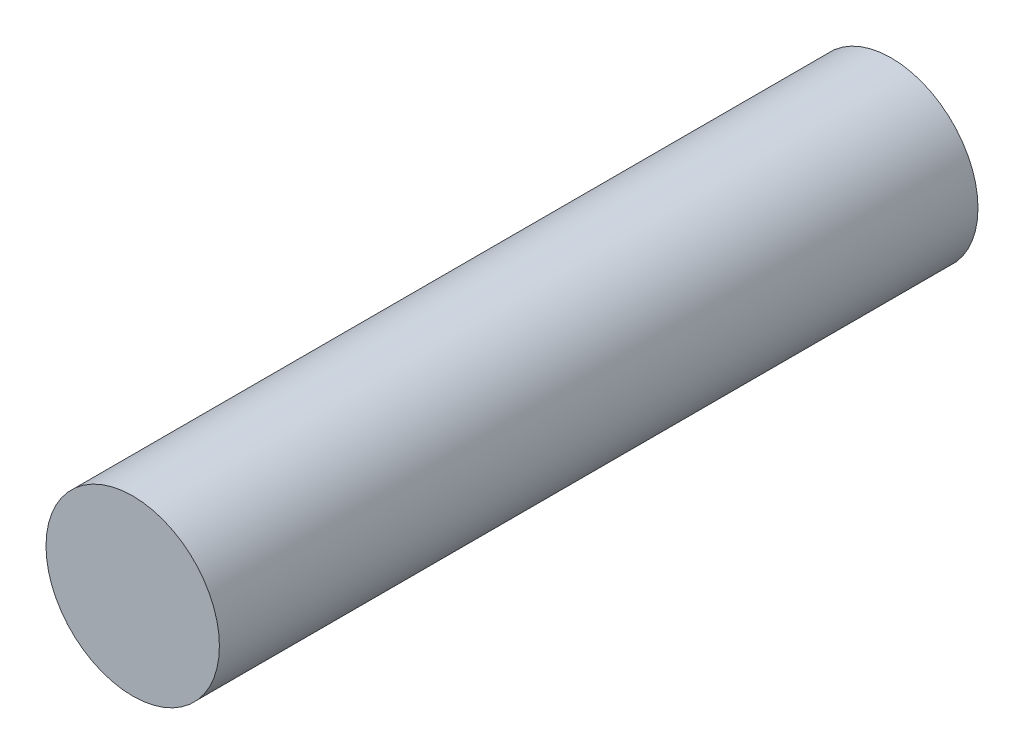
from build123d import *

# Parameters (mm, degrees)
SKETCH_1_R      = 4
EXTRUDE_1_DEPTH = 35


with BuildPart() as part:
    # 草图1 → 凸台-拉伸1 (new body)
    with BuildSketch(Plane.XY):
        Circle(SKETCH_1_R)
    extrude(amount=EXTRUDE_1_DEPTH)


solid = part.part
